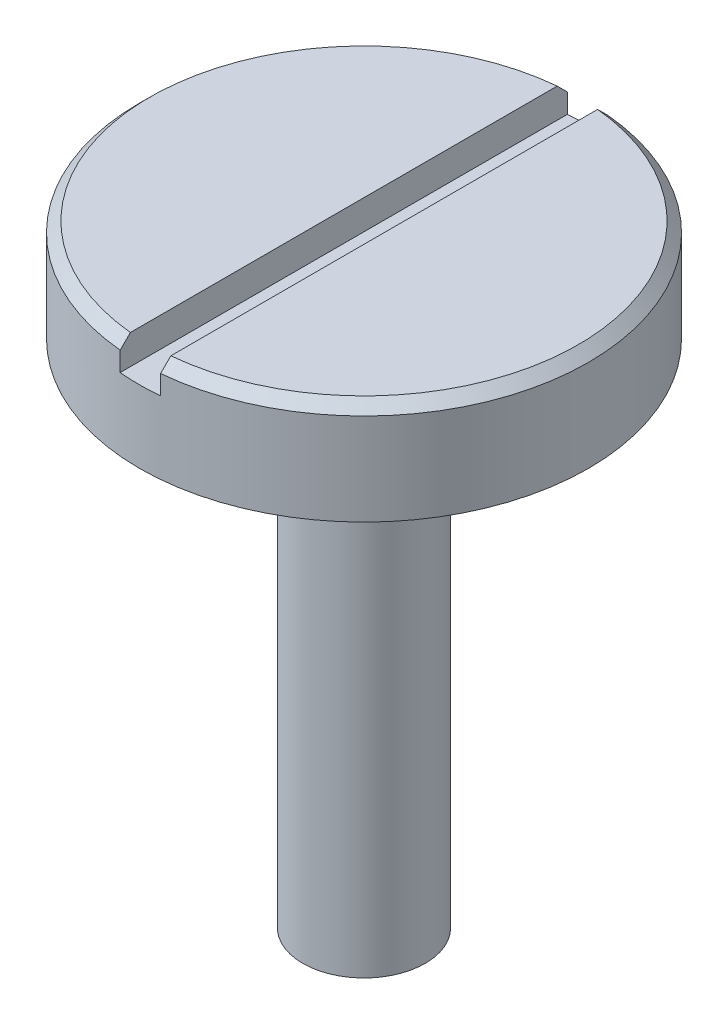
from build123d import *

# Parameters (mm, degrees)
SKETCH2_W          = 1.97993319
SKETCH2_H          = 2.899664475
CUT_EXTRUDE1_DEPTH = 18
CHAMFER1_SIZE      = 0.5


with BuildPart() as part:
    # Sketch1 → Revolve1 (revolve)
    with BuildSketch(Plane.XY, mode=Mode.PRIVATE) as revolve1_sk:
        Polygon((0, 21.201861416), (-11, 21.201861416), (-11, 16.201861416), (-3, 16.201861416), (-3, -8.798138584), (0, -8.798138584), align=None)
    revolve(revolve1_sk.sketch.rotate(Axis((0, 28.350797586, 0), (0, -1, 0)), 270), axis=Axis((0, 28.350797586, 0), (0, -1, 0)))

    # Sketch2 → Cut-Extrude1 (cut, symmetric)
    with BuildSketch(Plane.XY):
        with Locations((0, 21.201861416)):
            Rectangle(SKETCH2_W, SKETCH2_H)
    extrude(amount=CUT_EXTRUDE1_DEPTH, both=True, mode=Mode.SUBTRACT)

    # Chamfer1
    chamfer1_edges = [part.edges().sort_by_distance(p)[0] for p in [
        (-11, 21.201861416, 0),
        (11, 21.201861416, 0),
    ]]
    chamfer(chamfer1_edges, length=CHAMFER1_SIZE)


solid = part.part
